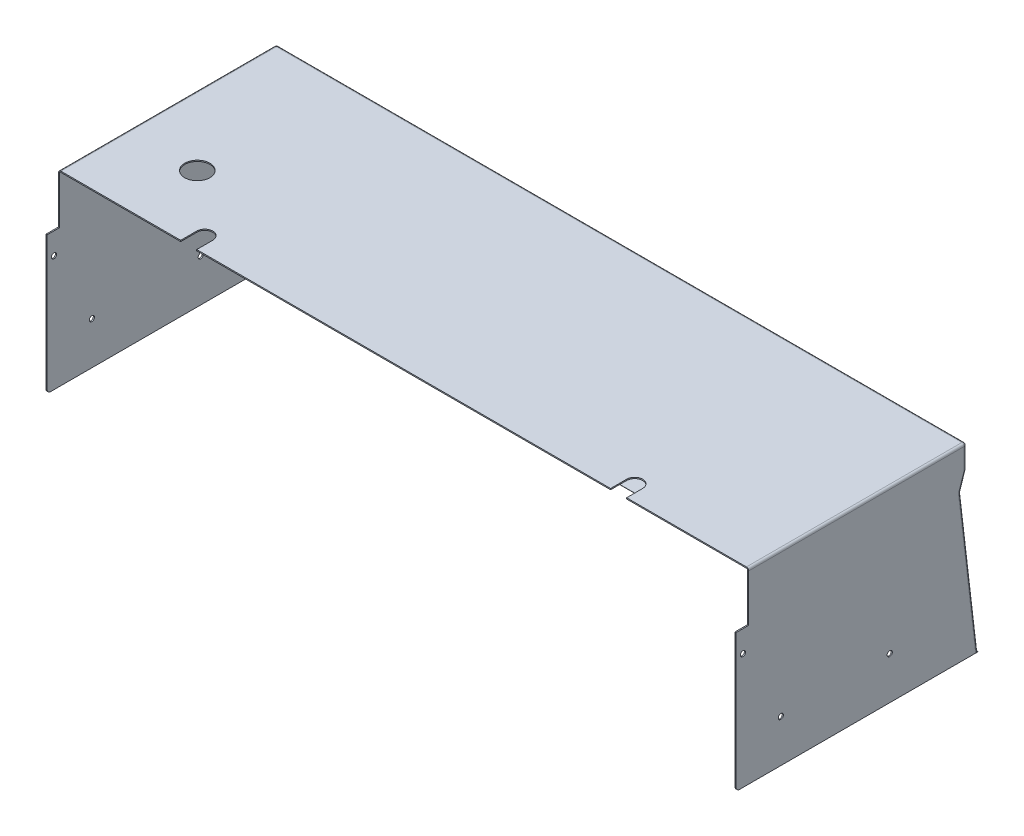
from build123d import *

# Parameters (mm, degrees)
EXTRUDE_1_DEPTH      = 301
EXTRUDE_1_2_DEPTH    = 1
SKETCH_8_R           = 11
CUT_EXTRUDE_3_DEPTH  = 2
SKETCH_12_R          = 12.5
CUT_EXTRUDE_6_DEPTH  = 397.494586373
SKETCH_13_W          = 602
SKETCH_13_H          = 30
EXTRUDE_5_DEPTH      = 0.15
SKETCH_14_R          = 2.25
CUT_EXTRUDE_7_DEPTH  = 655.989280083
FILLET_1_R           = 2
CUT_EXTRUDE_8_DEPTH  = 397.494586373
SKETCH_16_R          = 2.75
SKETCH_16_W          = 54
SKETCH_16_H          = 82
CUT_EXTRUDE_9_DEPTH  = 400.921435854
SKETCH_17_R          = 4
SKETCH_17_R_2        = 8
SKETCH_17_W          = 22
SKETCH_17_H          = 28.5
CUT_EXTRUDE_11_DEPTH = 10
FILLET_2_R           = 3
FILLET_3_R           = 3
SKETCH_19_R          = 11
CUT_EXTRUDE_12_DEPTH = 401.443879104


with BuildPart() as part:
    # 草图2 → Extrude 1 (new, symmetric)
    with BuildSketch(Plane(origin=(0, 0, 0), x_dir=(0, 0, -1), z_dir=(1, 0, 0))):
        Polygon((0, 0), (190, 0), (190, -20), (185, -35), (200, -163), (199.006796533, -163.116391031), (183.980866623, -34.895122471), (189, -19.83772234), (189, -1), (0, -1), align=None)
    extrude(amount=EXTRUDE_1_DEPTH, both=True)

    # 草图5 → Extrude 1 2 (add)
    with BuildSketch(Plane(origin=(301, 0, 0), x_dir=(0, 0, -1), z_dir=(1, 0, 0))):
        Polygon((0, -1), (189, -1), (189, -19.83772234), (183.980866623, -34.895122471), (199.006796533, -163.116391031), (-0.993203467, -163.116391031), (-10.993203467, -163.116391031), (-10.993203467, -43.116391031), (0, -43.116391031), align=None)
    extrude_1_2 = extrude(amount=-EXTRUDE_1_2_DEPTH)

    # 镜向1: Extrude 1 2 across plane
    add(extrude_1_2.mirror(Plane(origin=(0, 0, 0), x_dir=(0, 0, 1), z_dir=(1, 0, 0))))

    # 草图8 → 切除-拉伸3 (cut)
    with BuildSketch(Plane(origin=(0, 0, 0), x_dir=(-1, 0, 0), z_dir=(0, 1, 0))):
        with Locations(Location((240, -60, 0), (0, 0, 90))):
            Circle(SKETCH_8_R)
    extrude(amount=-CUT_EXTRUDE_3_DEPTH, mode=Mode.SUBTRACT)

    # 草图12 → 切除-拉伸6 (cut, through all)
    with BuildSketch(Plane.XY):
        with Locations(Location((-224, -93, 0), (0, 0, 90))):
            Circle(SKETCH_12_R)
    extrude(amount=-CUT_EXTRUDE_6_DEPTH, mode=Mode.SUBTRACT)

    # 草图13 → 凸台-拉伸5 (add)
    with BuildSketch(Plane.XZ.offset(163.116391031)):
        with Locations((0, -185)):
            Rectangle(SKETCH_13_W, SKETCH_13_H)
    extrude(amount=-EXTRUDE_5_DEPTH)

    # 草图14 → 切除-拉伸7 (cut, through all)
    with BuildSketch(Plane(origin=(301, 0, 0), x_dir=(0, 0, -1), z_dir=(1, 0, 0))):
        with Locations((-5, -62)):
            Circle(SKETCH_14_R)
        with Locations((28, -126)):
            Circle(SKETCH_14_R)
        with Locations((123, -126)):
            Circle(SKETCH_14_R)
    extrude(amount=-CUT_EXTRUDE_7_DEPTH, mode=Mode.SUBTRACT)

    # 圆角1
    fillet_1_edges = [part.edges().sort_by_distance(p)[0] for p in [
        (301, -98.983195516, -192.498030724),
        (-301, -98.983195516, -192.498030724),
        (301, -27.5, -187.5),
        (0, 0, -190),
        (0, -20, -190),
        (0, -35, -185),
        (301, -10, -190),
        (301, 0, -95),
        (-301, 0, -95),
        (-301, -10, -190),
        (-301, -27.5, -187.5),
    ]]
    fillet(fillet_1_edges, radius=FILLET_1_R)

    # 草图15 → 切除-拉伸8 (cut, through all)
    with BuildSketch(Plane(origin=(0, 0, 0), x_dir=(1, 0, 0), z_dir=(0, 1, 0))):
        with BuildLine():
            Line((180.5, 14), (180.5, -0.70941875))
            Line((180.5, -0.70941875), (194.5, -0.70941875))
            Line((194.5, -0.70941875), (194.5, 14))
            ThreePointArc((194.5, 14), (187.5, 21), (180.5, 14))
        make_face()
        with BuildLine():
            Line((-194.5, 14), (-194.5, -1.619416497))
            Line((-194.5, -1.619416497), (-180.5, -1.619416497))
            Line((-180.5, -1.619416497), (-180.5, 14))
            ThreePointArc((-180.5, 14), (-187.5, 21), (-194.5, 14))
        make_face()
    extrude(amount=-CUT_EXTRUDE_8_DEPTH, mode=Mode.SUBTRACT)

    # 草图16 → 切除-拉伸9 (cut, through all)
    with BuildSketch(Plane(origin=(0, 20.795463987, -177.454626023), x_dir=(1, 0, 0), z_dir=(0, -0.11639103134578274, 0.9932034674840121))):
        with Locations(Location((-111, -163.907896051, 0), (0, 0, 270))):
            Circle(SKETCH_16_R)
        with Locations(Location((-111, -73.907896051, 0), (0, 0, 270))):
            Circle(SKETCH_16_R)
        with Locations((-111, -119.740027582)):
            Rectangle(SKETCH_16_W, SKETCH_16_H)
    extrude(amount=-CUT_EXTRUDE_9_DEPTH, mode=Mode.SUBTRACT)

    # 草图17 → 切除-拉伸11 (cut)
    with BuildSketch(Plane(origin=(0, 20.911855018, -178.44782949), x_dir=(-1, 0, 0), z_dir=(0, 0.11639103134578274, -0.9932034674840121))):
        with Locations(Location((-7, -120.938280048, 0), (0, 0, 90))):
            Circle(SKETCH_17_R)
        with Locations(Location((33, -120.938280048, 0), (0, 0, 90))):
            Circle(SKETCH_17_R)
        with Locations(Location((-47, -120.938280048, 0), (0, 0, 90))):
            Circle(SKETCH_17_R_2)
        with Locations((-150, -120.938280048)):
            Rectangle(SKETCH_17_W, SKETCH_17_H)
        with Locations((-93, -120.938280048)):
            Rectangle(SKETCH_17_W, SKETCH_17_H)
    extrude(amount=-CUT_EXTRUDE_11_DEPTH, mode=Mode.SUBTRACT)

    # 圆角2
    fillet_2_edges = [part.edges().sort_by_distance(p)[0] for p in [
        (-300.5, -163.116391031, 10.993203467),
    ]]
    fillet(fillet_2_edges, radius=FILLET_2_R)

    # 圆角3
    fillet_3_edges = [part.edges().sort_by_distance(p)[0] for p in [
        (300.5, -163.116391031, 10.993203467),
    ]]
    fillet(fillet_3_edges, radius=FILLET_3_R)

    # 草图19 → 切除-拉伸12 (cut, through all)
    with BuildSketch(Plane(origin=(0, 20.911855018, -178.44782949), x_dir=(-1, 0, 0), z_dir=(0, 0.11639103134578274, -0.993203467484012))):
        with Locations(Location((-231, -120.938280048, 0), (0, 0, 90))):
            Circle(SKETCH_19_R)
    extrude(amount=-CUT_EXTRUDE_12_DEPTH, mode=Mode.SUBTRACT)


solid = part.part
